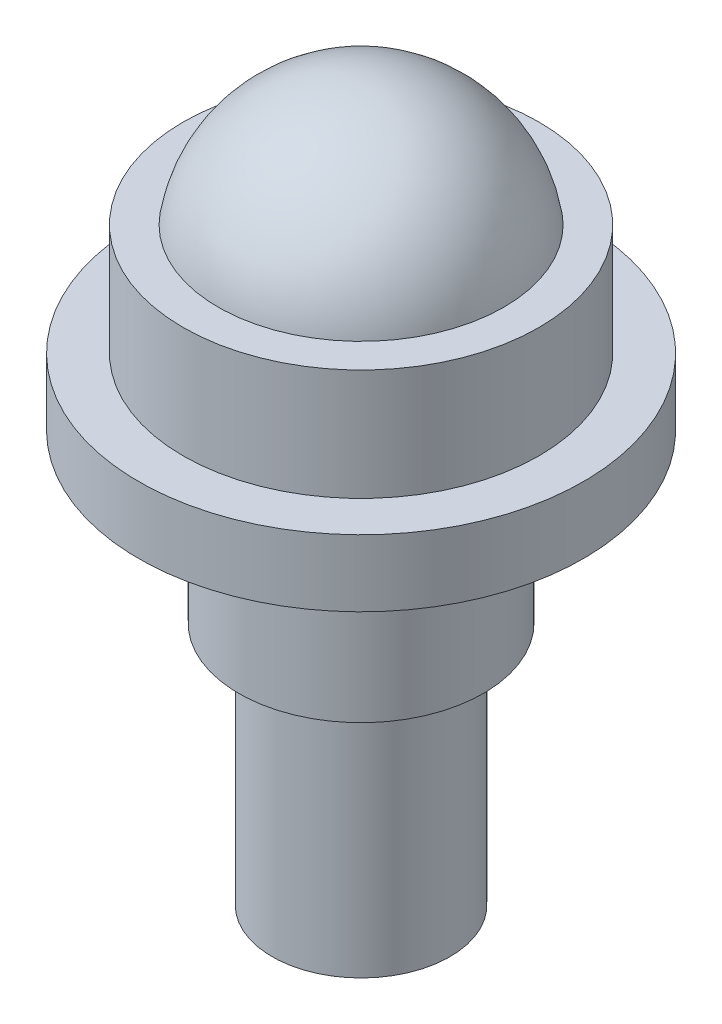
SolidWorks part; units mm, degrees
material "AISI 1015 钢，冷拔 (SS)"
ref_plane "Front Plane" through (0, 0, 0) normal (0, 0, 1) x (1, 0, 0)
ref_plane "Top Plane" through (0, 0, 0) normal (0, 1, 0) x (1, 0, 0)
ref_plane "Right Plane" through (0, 0, 0) normal (1, 0, 0) x (0, 0, -1)
other "Configuration Table"
sketch "Sketch1" plane through (0, 0, 0) normal (0, 0, 1) x (1, 0, 0)
  line L0 (0, 0) -> (0, 59.0607) construction
  line L1 (-12.8452, 16) -> (-16, 16)
  line L2 (-16, 16) -> (-16, 6)
  line L3 (-16, 6) -> (-20, 6)
  line L4 (-20, 6) -> (-20, 0)
  line L5 (-20, 0) -> (0, 0)
  line L6 (0, 0) -> (0, 27)
  arc A0 (0, 27) -> (-12.8452, 16) centre (0, 14) ccw
  dimension "D6" = 13
  dimension "D1" = 10
  dimension "D2" = 6
  dimension "D3" = 20
  dimension "D4" = 16
  dimension "D5" = 11
revolve "Revolve1" add sketch "Sketch1" angle 360 about L0
sketch "Sketch2" plane through (0, 0, 0) normal (0, -1, 0) x (-1, 0, 0)
  circle A0 centre (0, 0) radius 11
  dimension "D1" = 22
extrude "Boss-Extrude1" add sketch "Sketch2" along normal blind 15
sketch "Sketch3" plane through (0, -15, 0) normal (0, -1, 0) x (-1, 0, 0)
  circle A0 centre (0, 0) radius 8
  dimension "D1" = 16
extrude "Boss-Extrude2" add sketch "Sketch3" along normal blind 22
